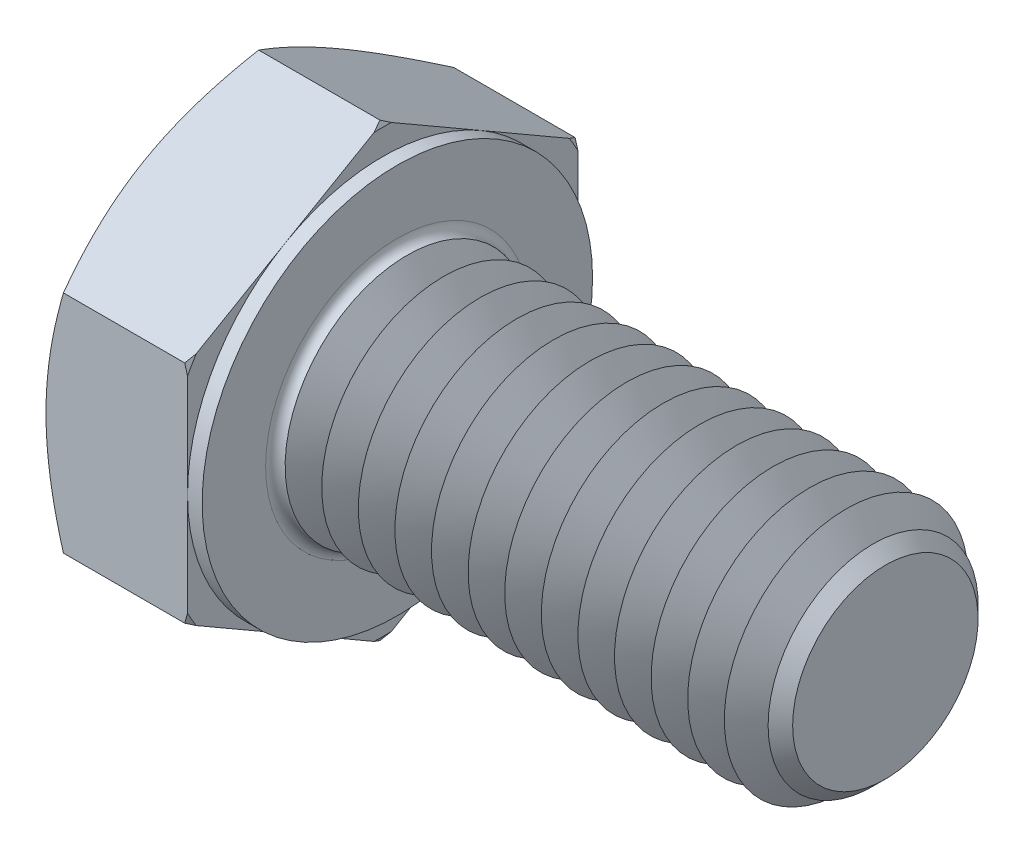
from build123d import *

# Parameters (mm, degrees)
BOSS_EXTRUDE_DEPTH = 6.4
SKETCH4_W          = 0.6
SKETCH4_H          = 11.237604307
CHAMFER_2_SIZE     = 1.2
FILLET_2_R         = 0.4
LPATTERN1_COUNT    = 13
LPATTERN1_PITCH    = 1.5


with BuildPart() as part:
    # Sketch1 → Boss-Extrude (new body)
    with BuildSketch(Plane(origin=(0, 0, 0), x_dir=(0, 0, -1), z_dir=(1, 0, 0))):
        Polygon((8, 4.618802154), (8, -4.618802154), (0, -9.237604307), (-8, -4.618802154), (-8, 4.618802154), (0, 9.237604307), align=None)
    extrude(amount=BOSS_EXTRUDE_DEPTH)

    # Sketch2 → Boss-Revolve1 (revolve)
    with BuildSketch(Plane.XY, mode=Mode.PRIVATE) as boss_revolve1_sk:
        Polygon((0, 0), (26.4, 0), (26.4, 3.701), (26.4, 5), (0, 5), align=None)
    revolve(boss_revolve1_sk.sketch.rotate(Axis((0, 0, 0), (1, 0, 0)), 90), axis=Axis((0, 0, 0), (1, 0, 0)))

    # Sketch3 → Cut-Revolve1 (revolve, cut)
    with BuildSketch(Plane.XY):
        Polygon((0, 8), (3.601282526, 14.237604307), (3.601282526, 19.237604307), (-10, 19.237604307), (-10, 8), align=None)
    revolve(axis=Axis((0, 0, 0), (1, 0, 0)), mode=Mode.SUBTRACT)

    # Sketch5 → Cut-Revolve2 (revolve, cut)
    with BuildSketch(Plane.XY):
        Polygon((6.4, 8), (2.798717474, 14.237604307), (2.798717474, 19.237604307), (12.798717474, 19.237604307), (12.798717474, 8), align=None)
    revolve(axis=Axis((0, 0, 0), (1, 0, 0)), mode=Mode.SUBTRACT)

    # Sketch4 → Cut-Revolve3 (revolve, cut)
    with BuildSketch(Plane.XY, mode=Mode.PRIVATE) as cut_revolve3_sk:
        with Locations((6.1, 13.618802154)):
            Rectangle(SKETCH4_W, SKETCH4_H)
    revolve(cut_revolve3_sk.sketch.rotate(Axis((0, 0, 0), (1, 0, 0)), 270), axis=Axis((0, 0, 0), (1, 0, 0)), mode=Mode.SUBTRACT)

    # Chamfer 2
    chamfer_2_edges = [part.edges().sort_by_distance(p)[0] for p in [
        (26.4, 0, -5),
    ]]
    chamfer(chamfer_2_edges, length=CHAMFER_2_SIZE)

    # Fillet 2
    fillet_2_edges = [part.edges().sort_by_distance(p)[0] for p in [
        (6.4, 0, -5),
    ]]
    fillet(fillet_2_edges, radius=FILLET_2_R)

    # Sketch6 → Cut-Revolve4 (revolve, cut)
    with BuildSketch(Plane.XY):
        Polygon((7.549978, -3.701), (6.8, -5), (6.8, -6.25), (8.299955999, -6.25), (8.299955999, -5), align=None)
    cut_revolve4 = revolve(axis=Axis((-3.175, 0, 0), (1, 0, 0)), mode=Mode.SUBTRACT)

    # LPattern1: Cut-Revolve4 ×13
    with Locations(*[(i * LPATTERN1_PITCH, 0, 0) for i in range(1, LPATTERN1_COUNT)]):
        add(cut_revolve4, mode=Mode.SUBTRACT)


solid = part.part
